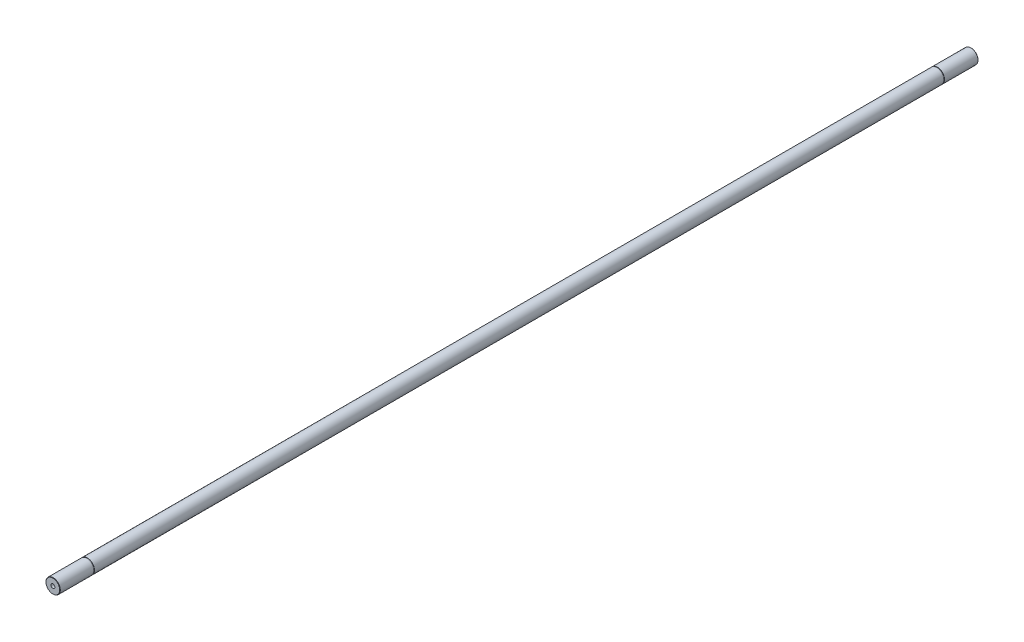
from build123d import *

# Parameters (mm, degrees)
SKETCH_1_R      = 12.5
EXTRUDE_1_DEPTH = 1600
CHAMFER_1_SIZE  = 0.5
SKETCH_2_W      = 0.55
SKETCH_2_H      = 1.3


with BuildPart() as part:
    # 草图1 → 凸台-拉伸1 (new body)
    with BuildSketch(Plane.XY):
        Circle(SKETCH_1_R)
    extrude(amount=EXTRUDE_1_DEPTH)

    # 倒角1
    chamfer_1_edges = [part.edges().sort_by_distance(p)[0] for p in [
        (-12.5, 0, 0),
        (-12.5, 0, 1600),
    ]]
    chamfer(chamfer_1_edges, length=CHAMFER_1_SIZE)

    # 草图2 → 切除-旋转1 (revolve, cut)
    with BuildSketch(Plane(origin=(0, 0, 0), x_dir=(1, 0, 0), z_dir=(0, 1, 0))):
        with Locations((12.225, -1540.55)):
            Rectangle(SKETCH_2_W, SKETCH_2_H)
    cut_revolve_1 = revolve(axis=Axis((0, 0, 1599.5), (0, 0, -1)), mode=Mode.SUBTRACT)

    # 草图5 → M8 螺纹孔1 (revolve, cut)
    with BuildSketch(Plane(origin=(0, 0, 1600), x_dir=(0, -1, 0), z_dir=(1, 0, 0))):
        Polygon((0, 0), (0, 21.792926105), (3.4, 19.75), (3.4, 0), align=None)
    hole_wizard_m8_1 = revolve(axis=Axis((0, 0, 1606.35), (0, 0, -1)), mode=Mode.SUBTRACT)

    # 镜向1: 切除-旋转1, M8 螺纹孔1 across plane
    add(cut_revolve_1.mirror(Plane.XY.offset(800)), mode=Mode.SUBTRACT)
    add(hole_wizard_m8_1.mirror(Plane.XY.offset(800)), mode=Mode.SUBTRACT)


solid = part.part
